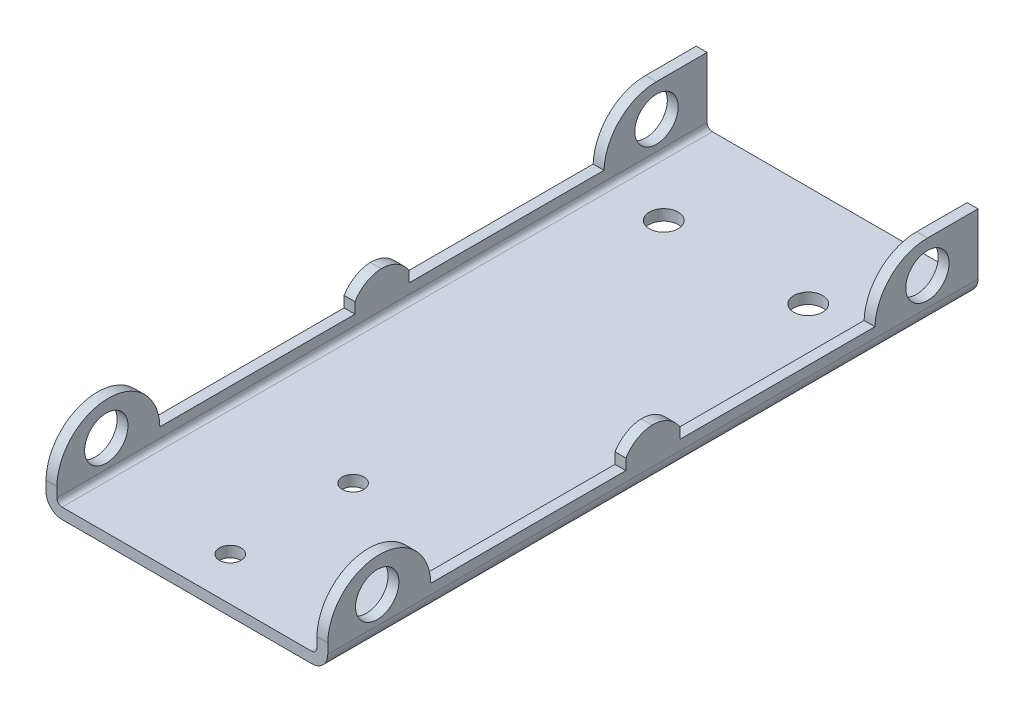
from build123d import *

# Parameters (mm, degrees)
BOSS_EXTRUDE1_DEPTH          = 1.5
SKETCH2_W                    = 90
SKETCH2_H                    = 1.5
BOSS_EXTRUDE2_DEPTH          = 36
BOSS_EXTRUDE3_DEPTH          = 1.5
F_6_0_6_DIAMETER_HOLE1_D     = 6
F_6_0_6_DIAMETER_HOLE1_DEPTH = 1.5
F_6_0_6_DIAMETER_HOLE2_D     = 6
F_4_0_4_DIAMETER_HOLE1_D     = 4
F_3_0_3_DIAMETER_HOLE1_D     = 3
FILLET1_R                    = 0.7366
FILLET2_R                    = 2.2366


with BuildPart() as part:
    # Sketch1 → Boss-Extrude1 (new body)
    with BuildSketch(Plane(origin=(-29, 0, 0), x_dir=(0, -1, 0), z_dir=(-1, 0, 0))):
        with BuildLine():
            Line((-9.138054181, -90), (1.5, -90))
            Line((1.5, -90), (1.5, 0))
            Line((1.5, 0), (-2.128893479, 0))
            ThreePointArc((-2.128893479, 0), (-9.130094082, -7.130859089), (-2.128893479, -14.261718178))
            Line((-2.128893479, -14.261718178), (-2.128893479, -41.261718178))
            Line((-2.128893479, -41.261718178), (-3.628893479, -41.261718178))
            ThreePointArc((-3.628893479, -41.261718178), (-5.147993713, -42.802982792), (-5.778257675, -44.873231442))
            ThreePointArc((-5.778257675, -44.873231442), (-5.210002115, -47.08061414), (-3.638283373, -48.73141787))
            Line((-3.638283373, -48.73141787), (-2.138054181, -48.73141787))
            Line((-2.138054181, -48.73141787), (-2.138054181, -75.73141787))
            ThreePointArc((-2.138054181, -75.73141787), (-7.103512649, -77.954400774), (-9.138054181, -83))
            Line((-9.138054181, -83), (-9.138054181, -90))
        make_face()
    extrude(amount=-BOSS_EXTRUDE1_DEPTH)

    # Sketch2 → Boss-Extrude2 (add)
    with BuildSketch(Plane(origin=(-27.5, 0, 0), x_dir=(0, 0, -1), z_dir=(1, 0, 0))):
        with Locations((45, -0.75)):
            Rectangle(SKETCH2_W, SKETCH2_H)
    extrude(amount=BOSS_EXTRUDE2_DEPTH)

    # Sketch3 → Boss-Extrude3 (add)
    with BuildSketch(Plane(origin=(8.5, 0, 0), x_dir=(0, 0, -1), z_dir=(1, 0, 0))):
        with BuildLine():
            Line((0, -1.5), (0, 2.128893479))
            ThreePointArc((0, 2.128893479), (7.130859089, 9.130094082), (14.261718178, 2.128893479))
            Line((14.261718178, 2.128893479), (41.261718178, 2.128893479))
            Line((41.261718178, 2.128893479), (41.261718178, 3.628893479))
            ThreePointArc((41.261718178, 3.628893479), (42.802982792, 5.147993713), (44.873231442, 5.778257675))
            ThreePointArc((44.873231442, 5.778257675), (47.08061414, 5.210002115), (48.73141787, 3.638283373))
            Line((48.73141787, 3.638283373), (48.73141787, 2.138054181))
            Line((48.73141787, 2.138054181), (75.73141787, 2.138054181))
            ThreePointArc((75.73141787, 2.138054181), (77.954400774, 7.103512649), (83, 9.138054181))
            Line((83, 9.138054181), (90, 9.138054181))
            Line((90, 9.138054181), (90, -1.5))
            Line((90, -1.5), (0, -1.5))
        make_face()
    extrude(amount=BOSS_EXTRUDE3_DEPTH)

    # Ø6.0 (6) Diameter Hole1
    with Locations(Plane.ZY.offset(-8.5)):
        with Locations((-6.845764439, 4.481725402), (-83, 4.638054181)):
            Hole(F_6_0_6_DIAMETER_HOLE1_D / 2, depth=F_6_0_6_DIAMETER_HOLE1_DEPTH)

    # Ø6.0 (6) Diameter Hole2 (through all)
    with Locations(Plane(origin=(-27.5, 0, 0), x_dir=(0, 0, -1), z_dir=(1, 0, 0))):
        with Locations((83, 4.638054181), (6.845764439, 4.481725402)):
            Hole(F_6_0_6_DIAMETER_HOLE2_D / 2)

    # Ø4.0 (4) Diameter Hole1 (through all)
    with Locations(Plane(origin=(0, 0, 0), x_dir=(1, 0, 0), z_dir=(0, 1, 0))):
        with Locations((-19.5, 76), (0.5, 76)):
            Hole(F_4_0_4_DIAMETER_HOLE1_D / 2)

    # Ø3.0 (3) Diameter Hole1 (through all)
    with Locations(Plane(origin=(0, 0, 0), x_dir=(1, 0, 0), z_dir=(0, 1, 0))):
        with Locations((-9.5, 6), (-9.5, 23)):
            Hole(F_3_0_3_DIAMETER_HOLE1_D / 2)

    # Fillet1
    fillet1_edges = [part.edges().sort_by_distance(p)[0] for p in [
        (-27.5, 0, -45),
        (8.5, 0, -45),
    ]]
    fillet(fillet1_edges, radius=FILLET1_R)

    # Fillet2
    fillet2_edges = [part.edges().sort_by_distance(p)[0] for p in [
        (-29, -1.5, -45),
        (10, -1.5, -45),
    ]]
    fillet(fillet2_edges, radius=FILLET2_R)


solid = part.part
